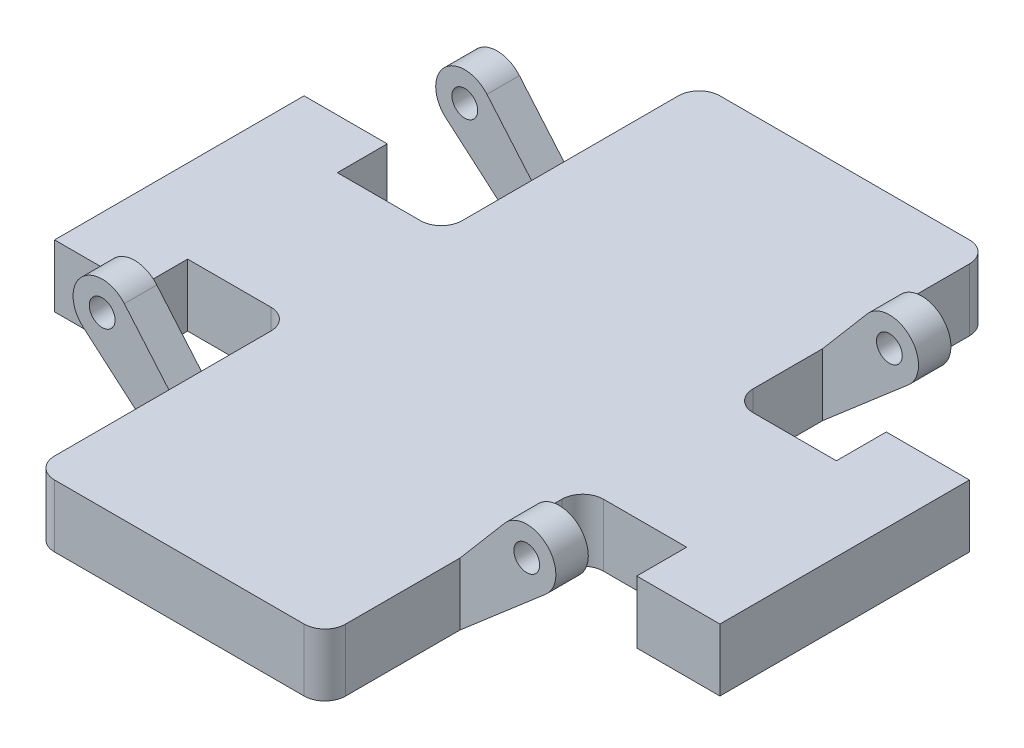
from build123d import *

# Parameters (mm, degrees)
SKETCH1_W               = 130
SKETCH1_H               = 130
BOSS_EXTRUDE1_DEPTH     = 15
SKETCH2_W               = 30
SKETCH2_H               = 30
CUT_EXTRUDE1_DEPTH      = 94.139680051
CUT_EXTRUDE4_START      = -10
SKETCH5_R               = 1.5
CUT_EXTRUDE4_DEPTH      = 84.139680051
SKETCH8_W               = 30
SKETCH8_H               = 17
CUT_EXTRUDE5_DEPTH      = 94.139680051
FILLET1_R               = 5
SKETCH9_W               = 70
SKETCH9_H               = 20
BOSS_EXTRUDE3_DEPTH     = 15
SKETCH10_R              = 3.1
BOSS_EXTRUDE4_DEPTH     = 3.9
MIRROR2_COPY_1_SKETCH_R = 3.1
MIRROR2_COPY_1_DEPTH    = 3.9
FILLET2_R               = 5
SKETCH7_W               = 20
SKETCH7_H               = 60
BOSS_EXTRUDE2_DEPTH     = 15


with BuildPart() as part:
    # Sketch1 → Boss-Extrude1 (new body)
    with BuildSketch(Plane(origin=(0, 0, 0), x_dir=(1, 0, 0), z_dir=(0, 1, 0))):
        Rectangle(SKETCH1_W, SKETCH1_H)
    extrude(amount=BOSS_EXTRUDE1_DEPTH)

    # Sketch2 → Cut-Extrude1 (cut, through all)
    with BuildSketch(Plane(origin=(0, 15, 0), x_dir=(1, 0, 0), z_dir=(0, 1, 0))):
        with Locations((-50, -50)):
            Rectangle(SKETCH2_W, SKETCH2_H)
        with Locations((-50, 50)):
            Rectangle(SKETCH2_W, SKETCH2_H)
        with Locations((50, 50)):
            Rectangle(SKETCH2_W, SKETCH2_H)
        with Locations((50, -50)):
            Rectangle(SKETCH2_W, SKETCH2_H)
    extrude(amount=-CUT_EXTRUDE1_DEPTH, mode=Mode.SUBTRACT)

    # Sketch5 → Cut-Extrude4 (cut, through all)
    with BuildSketch(Plane(origin=(0, 15, 0), x_dir=(1, 0, 0), z_dir=(0, 1, 0)).offset(CUT_EXTRUDE4_START)):
        with Locations(Location((-38.5, 0, 0), (0, 0, 270))):
            Circle(SKETCH5_R)
        with Locations(Location((-58.5, 0, 0), (0, 0, 270))):
            Circle(SKETCH5_R)
        with Locations(Location((-48.5, 10, 0), (0, 0, 270))):
            Circle(SKETCH5_R)
        with Locations(Location((-48.5, -10, 0), (0, 0, 270))):
            Circle(SKETCH5_R)
        with Locations(Location((10, 48.5, 0), (0, 0, 270))):
            Circle(SKETCH5_R)
        with Locations(Location((0, 38.5, 0), (0, 0, 270))):
            Circle(SKETCH5_R)
        with Locations(Location((-10, 48.5, 0), (0, 0, 270))):
            Circle(SKETCH5_R)
        with Locations(Location((0, 58.5, 0), (0, 0, 270))):
            Circle(SKETCH5_R)
        with Locations(Location((48.5, -10, 0), (0, 0, 270))):
            Circle(SKETCH5_R)
        with Locations(Location((38.5, 0, 0), (0, 0, 270))):
            Circle(SKETCH5_R)
        with Locations(Location((48.5, 10, 0), (0, 0, 270))):
            Circle(SKETCH5_R)
        with Locations(Location((58.5, 0, 0), (0, 0, 270))):
            Circle(SKETCH5_R)
        with Locations(Location((-10, -48.5, 0), (0, 0, 270))):
            Circle(SKETCH5_R)
        with Locations(Location((0, -38.5, 0), (0, 0, 270))):
            Circle(SKETCH5_R)
        with Locations(Location((10, -48.5, 0), (0, 0, 270))):
            Circle(SKETCH5_R)
        with Locations(Location((0, -58.5, 0), (0, 0, 270))):
            Circle(SKETCH5_R)
    extrude(amount=-CUT_EXTRUDE4_DEPTH, mode=Mode.SUBTRACT)

    # Sketch8 → Cut-Extrude5 (cut, through all)
    with BuildSketch(Plane(origin=(0, 15, 0), x_dir=(1, 0, 0), z_dir=(0, 1, 0))):
        with Locations((50, 26.5)):
            Rectangle(SKETCH8_W, SKETCH8_H)
        with Locations((50, -26.5)):
            Rectangle(SKETCH8_W, SKETCH8_H)
        with Locations((-50, 26.5)):
            Rectangle(SKETCH8_W, SKETCH8_H)
        with Locations((-50, -26.5)):
            Rectangle(SKETCH8_W, SKETCH8_H)
    extrude(amount=-CUT_EXTRUDE5_DEPTH, mode=Mode.SUBTRACT)

    # Fillet1
    fillet1_edges = [part.edges().sort_by_distance(p)[0] for p in [
        (35, 7.5, 18),
        (65, 7.5, 18),
        (-35, 7.5, -18),
        (-65, 7.5, -18),
        (-35, 7.5, 18),
        (-65, 7.5, 18),
        (35, 7.5, -18),
        (65, 7.5, -18),
        (35, 7.5, 65),
        (35, 7.5, -65),
        (-35, 7.5, -65),
        (-35, 7.5, 65),
    ]]
    fillet(fillet1_edges, radius=FILLET1_R)

    # Sketch9 → Boss-Extrude3 (add)
    with BuildSketch(Plane(origin=(0, 15, 0), x_dir=(1, 0, 0), z_dir=(0, 1, 0))):
        with Locations((0, 70)):
            Rectangle(SKETCH9_W, SKETCH9_H)
        with Locations((0, -70)):
            Rectangle(SKETCH9_W, SKETCH9_H)
    extrude(amount=-BOSS_EXTRUDE3_DEPTH)

    # Sketch10 → Boss-Extrude4 (add, symmetric)
    with BuildSketch(Plane(origin=(0, 0, -43.6), x_dir=(-1, 0, 0), z_dir=(0, 0, -1))):
        with BuildLine():
            Line((35, 15), (45.716265876, 27.602517314))
            ThreePointArc((45.716265876, 27.602517314), (55.982579723, 28.033806961), (55.61817193, 17.76490158))
            Line((55.61817193, 17.76490158), (35, 0))
            Line((35, 0), (35, 15))
        make_face()
        with Locations((51.048979422, 23.06796483)):
            Circle(SKETCH10_R, mode=Mode.SUBTRACT)
    boss_extrude4 = extrude(amount=BOSS_EXTRUDE4_DEPTH, both=True)

    # Mirror1: Boss-Extrude4 across plane
    add(boss_extrude4.mirror(Plane(origin=(0, 0, 0), x_dir=(0, 0, 1), z_dir=(1, 0, 0))))

    # Mirror2: Boss-Extrude4 across plane
    add(boss_extrude4.mirror(Plane.XY))

    # Mirror2 copy 1 sketch → Mirror2 copy 1 (add, symmetric)
    with BuildSketch(Plane.XY.offset(43.6)):
        with BuildLine():
            Line((35, 15), (45.716265876, 27.602517314))
            ThreePointArc((45.716265876, 27.602517314), (55.982579723, 28.033806961), (55.61817193, 17.76490158))
            Line((55.61817193, 17.76490158), (35, 0))
            Line((35, 0), (35, 15))
        make_face()
        with Locations((51.048979422, 23.06796483)):
            Circle(MIRROR2_COPY_1_SKETCH_R, mode=Mode.SUBTRACT)
    extrude(amount=MIRROR2_COPY_1_DEPTH, both=True)

    # Fillet2
    fillet2_edges = [part.edges().sort_by_distance(p)[0] for p in [
        (-35, 7.5, -80),
        (35, 7.5, -80),
        (-35, 7.5, 80),
        (35, 7.5, 80),
    ]]
    fillet(fillet2_edges, radius=FILLET2_R)

    # Sketch7 → Boss-Extrude2 (add)
    with BuildSketch(Plane(origin=(0, 15, 0), x_dir=(1, 0, 0), z_dir=(0, 1, 0))):
        with Locations((-70, 0)):
            Rectangle(SKETCH7_W, SKETCH7_H)
        with Locations((70, 0)):
            Rectangle(SKETCH7_W, SKETCH7_H)
    extrude(amount=-BOSS_EXTRUDE2_DEPTH)


solid = part.part
